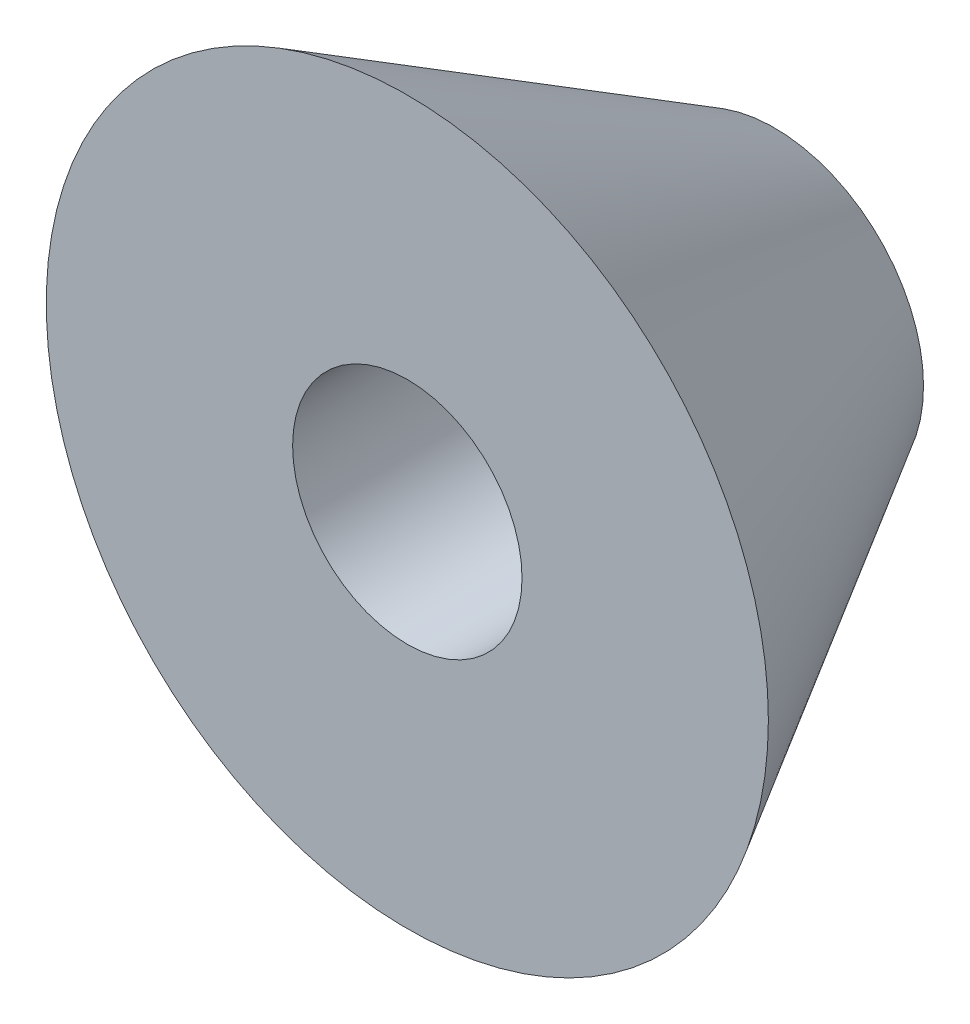
from build123d import *

# Parameters (mm, degrees)
SKETCH1_R           = 3.25
BOSS_EXTRUDE1_DEPTH = 8
BOSS_EXTRUDE1_DRAFT = -30
SKETCH2_R           = 2.5
CUT_EXTRUDE1_DEPTH  = 14.705330885


with BuildPart() as part:
    # Sketch1 → Boss-Extrude1 (with draft: the straight prism first)
    with BuildSketch(Plane.XY):
        Circle(SKETCH1_R)
    extrude(amount=BOSS_EXTRUDE1_DEPTH)
    # Boss-Extrude1: the draft: its side faces are tilted about the plane it starts from
    boss_extrude1_sides = [part.faces().sort_by_distance(p)[0] for p in [
        (-3.25, 0, 4),
    ]]
    draft(boss_extrude1_sides, Plane.XY, BOSS_EXTRUDE1_DRAFT)

    # Sketch2 → Cut-Extrude1 (cut, through all)
    with BuildSketch(Plane(origin=(0, 0, 0), x_dir=(-1, 0, 0), z_dir=(0, 0, -1))):
        Circle(SKETCH2_R)
    extrude(amount=-CUT_EXTRUDE1_DEPTH, mode=Mode.SUBTRACT)


solid = part.part
